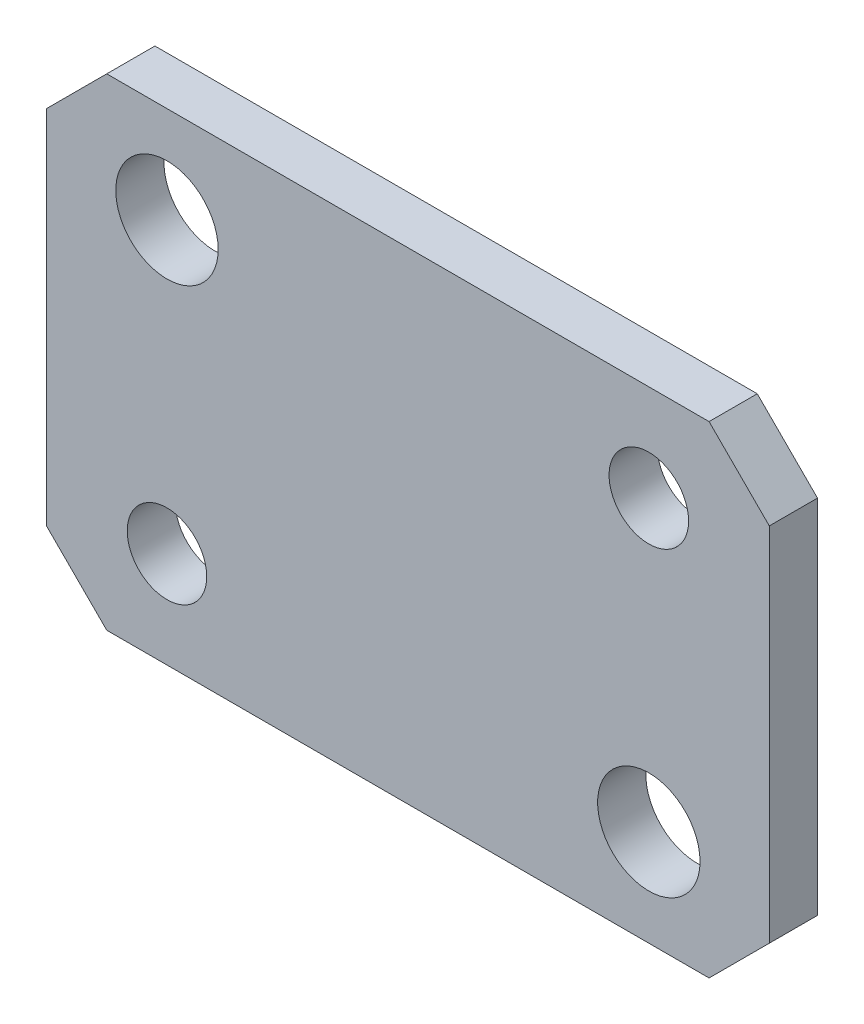
SolidWorks part; units mm, degrees
material "Q235-A"
ref_plane "Front Plane" through (0, 0, 0) normal (0, 0, 1) x (1, 0, 0)
ref_plane "Top Plane" through (0, 0, 0) normal (0, 1, 0) x (1, 0, 0)
ref_plane "Right Plane" through (0, 0, 0) normal (1, 0, 0) x (0, 0, -1)
sketch "Sketch1" plane through (0, 0, 0) normal (0, 0, 1) x (1, 0, 0)
  line L1 (-24.9905, 14.4664) -> (35.0095, 14.4664)
  line L2 (-24.9905, 14.4664) -> (-24.9905, -25.5336)
  line L3 (-24.9905, -25.5336) -> (35.0095, -25.5336)
  line L4 (35.0095, 14.4664) -> (35.0095, -25.5336)
  line L5 (-14.9905, 6.4664) -> (25.0095, 6.4664) construction
  line L6 (-14.9905, 6.4664) -> (-14.9905, -17.5336) construction
  line L7 (-14.9905, -17.5336) -> (25.0095, -17.5336) construction
  line L8 (25.0095, 6.4664) -> (25.0095, -17.5336) construction
  line L9 (-14.9905, 6.4664) -> (25.0095, -17.5336) construction
  line L10 (-14.9905, -17.5336) -> (25.0095, 6.4664) construction
  circle A0 centre (-14.9905, 6.4664) radius 4.25
  circle A1 centre (25.0095, -17.5336) radius 4.25
  circle A2 centre (25.0095, 6.4664) radius 3.3
  circle A3 centre (-14.9905, -17.5336) radius 3.3
  point P8 (5.0095, -5.5336)
  dimension "D1" = 60
  dimension "D2" = 40
  dimension "D3" = 40
  dimension "D4" = 24
  dimension "D5" = 8
  dimension "D6" = 10
extrude "Boss-Extrude1" add sketch "Sketch1" along normal blind 4
chamfer "Chamfer1" distance 5 angle 45 4 edges at (35.0095, 14.4664, 2) (35.0095, -25.5336, 2) (-24.9905, -25.5336, 2) (-24.9905, 14.4664, 2)
